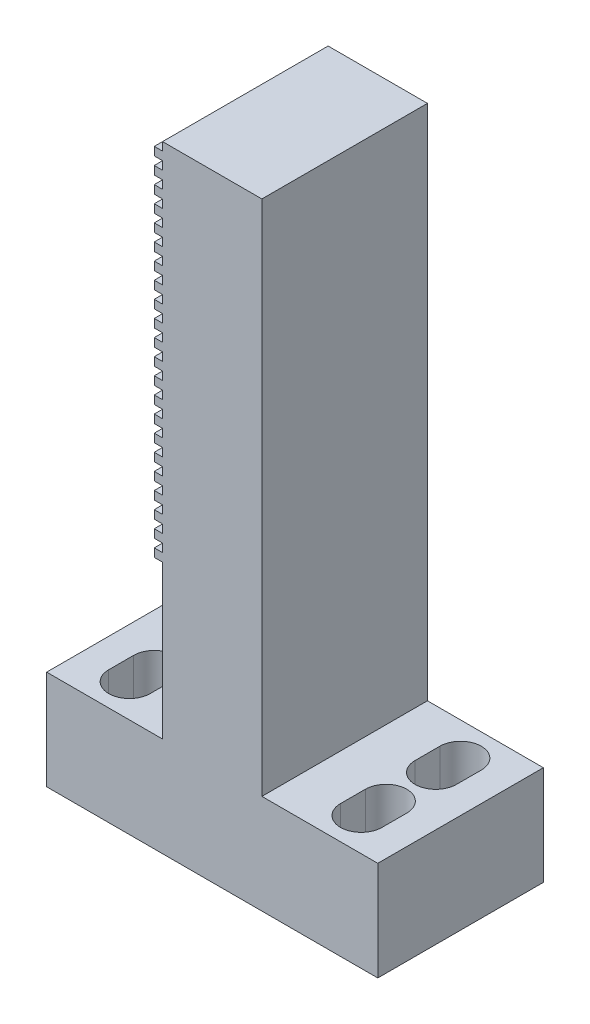
SolidWorks part; units mm, degrees
ref_plane "前视基准面" through (0, 0, 0) normal (0, 0, 1) x (1, 0, 0)
ref_plane "上视基准面" through (0, 0, 0) normal (0, 1, 0) x (1, 0, 0)
ref_plane "右视基准面" through (0, 0, 0) normal (1, 0, 0) x (0, 0, -1)
sketch "草图1" plane through (0, 0, 0) normal (0, 0, 1) x (1, 0, 0)
  line L0 (0, 0) -> (-20, 0)
  line L1 (-20, 0) -> (-20, 12)
  line L2 (-20, 12) -> (-6, 12)
  line L3 (-6, 12) -> (-6, 74.5)
  line L4 (-6, 74.5) -> (6, 74.5)
  line L5 (6, 74.5) -> (6, 12)
  line L6 (6, 12) -> (20, 12)
  line L7 (20, 12) -> (20, 0)
  line L8 (20, 0) -> (0, 0)
  dimension "D1" = 12
  dimension "D2" = 62.5
  dimension "D3" = 12
  dimension "D4" = 40
extrude "凸台-拉伸1" add sketch "草图1" along normal mid plane 20
sketch "草图2" plane through (0, 12, 0) normal (0, 1, 0) x (1, 0, 0)
  line L0 (-14, 3) -> (-14, 6) construction
  line L1 (-16.5, 3) -> (-16.5, 6)
  line L2 (-11.5, 3) -> (-11.5, 6)
  line L3 (-14, -6) -> (-14, -3) construction
  line L4 (-16.5, -6) -> (-16.5, -3)
  line L5 (-11.5, -6) -> (-11.5, -3)
  line L6 (-20, -10) -> (-20, 10) construction
  line L7 (-6, 10) -> (-20, 10) construction
  line L8 (-6, -10) -> (-20, -10) construction
  line L9 (0, 10) -> (0, -10) construction
  line L10 (6, 10) -> (-6, 10) construction
  line L11 (6, -10) -> (-6, -10) construction
  line L12 (14, -6) -> (14, -3) construction
  line L13 (16.5, -6) -> (16.5, -3)
  line L14 (11.5, -6) -> (11.5, -3)
  line L15 (14, 3) -> (14, 6) construction
  line L16 (16.5, 3) -> (16.5, 6)
  line L17 (11.5, 3) -> (11.5, 6)
  arc A0 (-16.5, 3) -> (-11.5, 3) centre (-14, 3) ccw
  arc A1 (-11.5, 6) -> (-16.5, 6) centre (-14, 6) ccw
  arc A2 (-16.5, -6) -> (-11.5, -6) centre (-14, -6) ccw
  arc A3 (-11.5, -3) -> (-16.5, -3) centre (-14, -3) ccw
  arc A4 (16.5, -6) -> (11.5, -6) centre (14, -6) cw
  arc A5 (11.5, -3) -> (16.5, -3) centre (14, -3) cw
  arc A6 (16.5, 3) -> (11.5, 3) centre (14, 3) cw
  arc A7 (11.5, 6) -> (16.5, 6) centre (14, 6) cw
  point P2 (-14, 4.5)
  point P8 (-14, -4.5)
  point P28 (14, -4.5)
  point P35 (14, 4.5)
extrude "切除-拉伸1" cut sketch "草图2" against normal up to next
sketch "草图3" plane through (-6, 0, 0) normal (-1, 0, 0) x (0, 0, 1)
  line L0 (-10, 74.5) -> (-10, 12) construction
  line L1 (-10, 73.5) -> (10, 73.5)
  line L2 (-10, 73.5) -> (-10, 72.5)
  line L3 (-10, 72.5) -> (10, 72.5)
  line L4 (10, 73.5) -> (10, 72.5)
  line L5 (10, 74.5) -> (10, 12) construction
  line L6 (10, 74.5) -> (-10, 74.5) construction
  dimension "D1" = 1
  dimension "D2" = 1
extrude "凸台-拉伸2" add sketch "草图3" along normal blind 1
pattern_linear "阵列(线性)1" count 22 spacing 2 along (0, -1, 0) of "凸台-拉伸2"
equation "\"D5@草图2\"=\"D4@草图2\""
